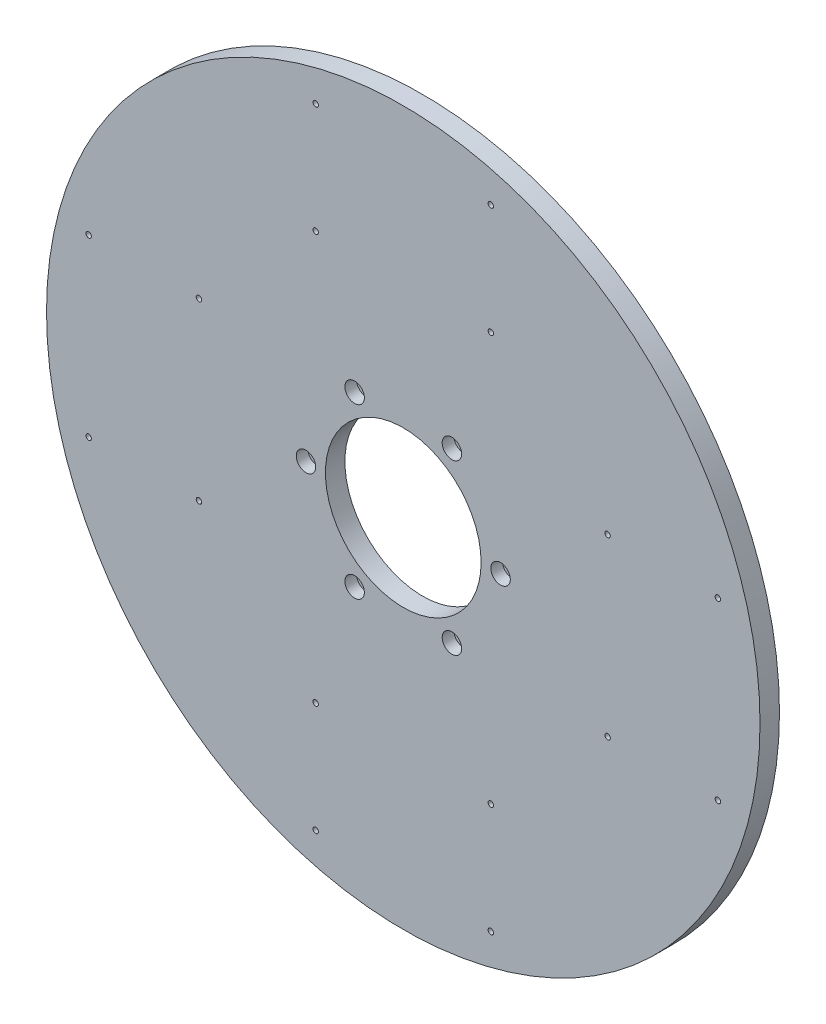
SolidWorks part; units mm, degrees
ref_plane "Front Plane" through (0, 0, 0) normal (0, 0, 1) x (1, 0, 0)
ref_plane "Top Plane" through (0, 0, 0) normal (0, 1, 0) x (1, 0, 0)
ref_plane "Right Plane" through (0, 0, 0) normal (1, 0, 0) x (0, 0, -1)
sketch "Sketch1" plane through (0, 0, 0) normal (0, 0, 1) x (1, 0, 0)
  circle A0 centre (0, 0) radius 275
  dimension "D1" = 550
extrude "Boss-Extrude1" add sketch "Sketch1" along normal blind 15
sketch "Sketch2" plane through (0, 0, 15) normal (0, 0, 1) x (1, 0, 0)
  circle A0 centre (0, 0) radius 60
  dimension "D1" = 120
extrude "Cut-Extrude1" cut sketch "Sketch2" against normal through all
hole_wizard "M5 Tapped Hole1" positions "Sketch13" profile "Sketch14" tap size "M5" standard "GB" end condition through all
sketch "Sketch13" plane through (0, 0, 15) normal (0, 0, 1) x (1, 0, 0)
  line L0 (67.5, 242.5) -> (67.5, 157.5) construction
  line L2 (35.4677, 200) -> (50035.4677, 200) construction
  line L4 (0, 0) -> (0, -50000) construction
  point P0 (67.5, 157.5)
  point P2 (67.5, 242.5)
  point P12 (67.5, 200)
  point P21 (-67.5, 157.5)
  point P22 (-67.5, 242.5)
  dimension "D1" = 85
  dimension "D2" = 200
  dimension "D3" = 135
sketch "Sketch14" plane through (67.5, 157.5, 15) normal (1, 0, 0) x (0, -1, 0)
  line L0 (0, 0) -> (0, 15)
  line L1 (0, 15) -> (2.1, 15)
  line L2 (2.1, 15) -> (2.1, 0)
  line L5 (2.1, 0) -> (0, 0)
  line L11 (0, -6.35) -> (0, 107.95) construction
  dimension "通孔螺纹孔钻头直径" = 4.2
  dimension "通孔螺纹孔钻头深度" = 15
cosmetic thread "Cosmetic Thread1" parameters "D2"=5
cosmetic thread "Cosmetic Thread2" parameters "D2"=5
cosmetic thread "Cosmetic Thread3" parameters "D2"=5
cosmetic thread "Cosmetic Thread4" parameters "D2"=5
pattern_circular "CirPattern1" count 4 over 360 about axis through (0, 0, 0) along (0, 0, 1) of "M5 Tapped Hole1"
hole_wizard "Hole Size (%based) Socket Head Cap Screw Type1" positions "Sketch17" profile "Sketch18" counterbore size "M8" standard "GB" end condition through all
sketch "Sketch17" plane through (0, 0, 15) normal (0, 0, 1) x (1, 0, 0)
  line L0 (0, 0) -> (50000, 0) construction
  line L1 (0, 0) -> (0, -50000) construction
  line L2 (0, 0) -> (-37.5, 64.9519) construction
  point P0 (-37.5, 64.9519)
  dimension "D1" = 75
  dimension "D2" = 60
sketch "Sketch18" plane through (-37.5, 64.9519, 15) normal (1, 0, 0) x (0, -1, 0)
  line L0 (0, 0) -> (0, 15)
  line L1 (0, 15) -> (4.5, 15)
  line L3 (4.5, 15) -> (4.5, 9)
  line L4 (4.5, 9) -> (7.5, 9)
  line L5 (7.5, 9) -> (7.5, 0)
  line L7 (7.5, 0) -> (0, 0)
  line L11 (0, -6.35) -> (0, 107.95) construction
  dimension "通孔孔直径" = 9
  dimension "通孔孔深度" = 15
  dimension "柱形沉头孔直径" = 15
  dimension "柱形沉头孔深度" = 9
pattern_circular "CirPattern2" count 6 over 360 about axis through (0, 0, 0) along (0, 0, 1) of "Hole Size (%based) Socket Head Cap Screw Type1"
